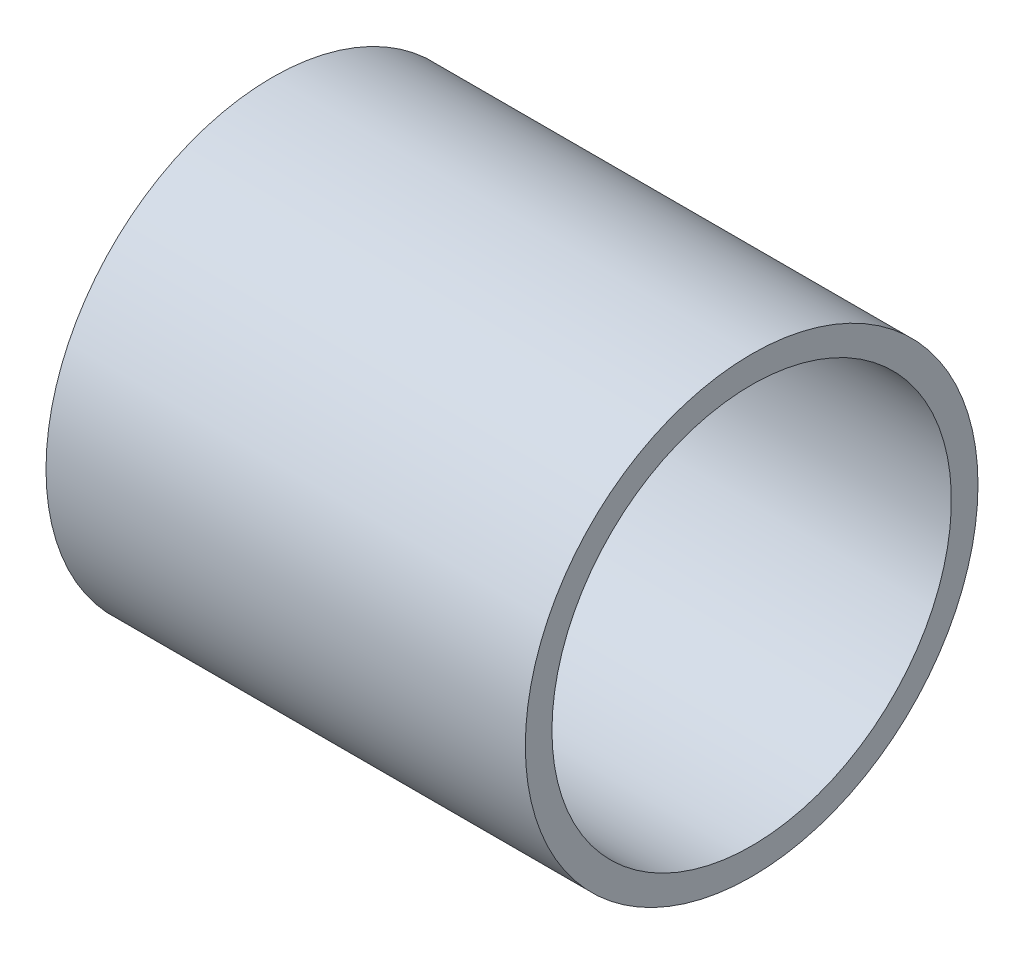
from build123d import *

# Parameters (mm, degrees)
SKETCH1_R           = 85
SKETCH1_R_2         = 75
BOSS_EXTRUDE1_DEPTH = 180


with BuildPart() as part:
    # Sketch1 → Boss-Extrude1 (new body)
    with BuildSketch(Plane(origin=(0, 0, 0), x_dir=(0, 0, -1), z_dir=(1, 0, 0))):
        with Locations(Location((0, 0, 0), (0, 0, 180))):
            Circle(SKETCH1_R)
        with Locations(Location((0, 0, 0), (0, 0, 180))):
            Circle(SKETCH1_R_2, mode=Mode.SUBTRACT)
    extrude(amount=BOSS_EXTRUDE1_DEPTH)


solid = part.part
